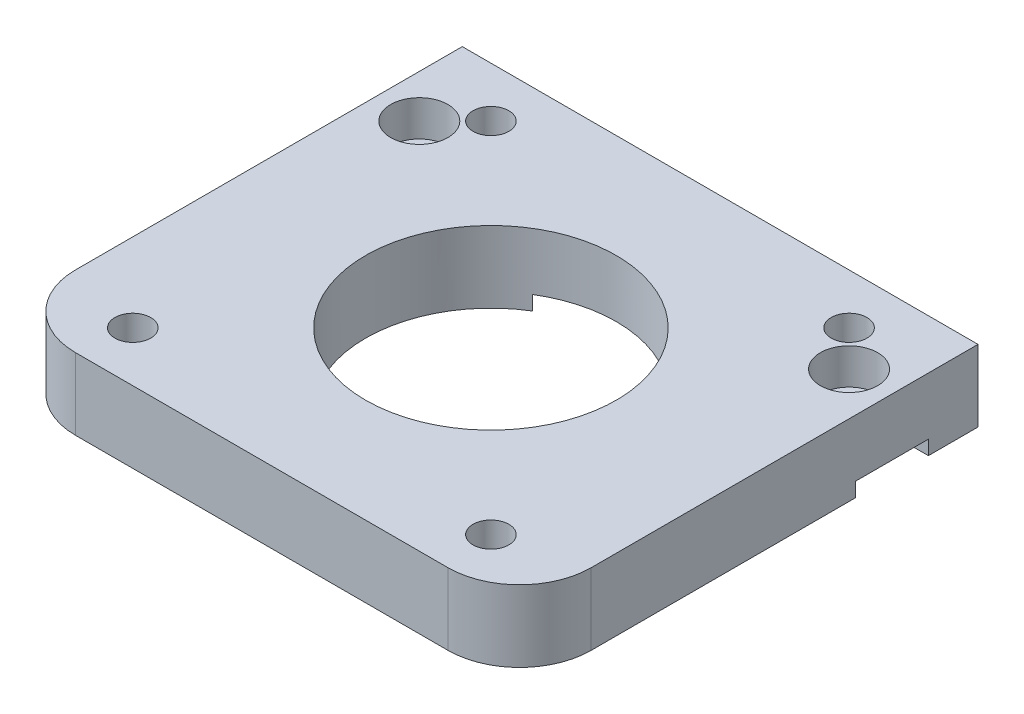
from build123d import *

# Parameters (mm, degrees)
SKETCH_1_W                = 103
SKETCH_1_H                = 100
EXTRUDE_1_DEPTH           = 10
SKETCH_9_W                = 15.5
SKETCH_9_H                = 88
CUT_EXTRUDE_4_DEPTH       = 144.906219463
HOLE_WIZARD_6_5_6_5_1_D   = 6.5
SKETCH_12_R               = 17.5
CUT_EXTRUDE_5_DEPTH       = 144.906219463
FILLET_1_R                = 10
HOLE_WIZARD_5_0_5_1_D     = 5
HOLE_WIZARD_5_0_5_1_DEPTH = 10
HOLE_WIZARD_5_0_5_1_TIP   = 1.502151548
FILLET_2_R                = 2
SKETCH_20_W               = 140.430498758
SKETCH_20_H               = 45.630669844
CUT_EXTRUDE_6_DEPTH       = 97
HOLE_WIZARD_1_D           = 4.4
HOLE_WIZARD_1_CBORE_D     = 8
HOLE_WIZARD_1_CBORE_DEPTH = 5
HOLE_WIZARD_M6_2_D        = 5
SKETCH_28_W               = 143.680703706
SKETCH_28_H               = 10.15
CUT_EXTRUDE_7_DEPTH       = 2


with BuildPart() as part:
    # 草图1 → 凸台-拉伸1 (new body)
    with BuildSketch(Plane(origin=(0, 0, 0), x_dir=(1, 0, 0), z_dir=(0, 1, 0))):
        with Locations((51.5, -50)):
            Rectangle(SKETCH_1_W, SKETCH_1_H)
    extrude(amount=EXTRUDE_1_DEPTH)

    # 草图9 → 切除-拉伸4 (cut, through all)
    with BuildSketch(Plane(origin=(0, 10, 0), x_dir=(1, 0, 0), z_dir=(0, 1, 0))):
        with Locations((7.75, -56)):
            Rectangle(SKETCH_9_W, SKETCH_9_H)
        with Locations((95.25, -56)):
            Rectangle(SKETCH_9_W, SKETCH_9_H)
    extrude(amount=-CUT_EXTRUDE_4_DEPTH, mode=Mode.SUBTRACT)

    # Ø6.5 (6.5) 直径孔1 (through all)
    with Locations(Plane.XY.offset(12)):
        with Locations((6, 5), (97, 5)):
            Hole(HOLE_WIZARD_6_5_6_5_1_D / 2)

    # 草图12 → 切除-拉伸5 (cut, through all)
    with BuildSketch(Plane(origin=(0, 10, 0), x_dir=(1, 0, 0), z_dir=(0, 1, 0))):
        with Locations(Location((51.5, -68, 0), (0, 0, 270))):
            Circle(SKETCH_12_R)
    extrude(amount=-CUT_EXTRUDE_5_DEPTH, mode=Mode.SUBTRACT)

    # 圆角1
    fillet_1_edges = [part.edges().sort_by_distance(p)[0] for p in [
        (15.5, 5, 100),
        (87.5, 5, 100),
    ]]
    fillet(fillet_1_edges, radius=FILLET_1_R)

    # Ø5.0 (5) 直径孔1
    with Locations(Plane(origin=(0, 0, 0), x_dir=(-1, 0, 0), z_dir=(0, 0, -1))):
        with Locations((-71.5, 5), (-31.5, 5)):
            Hole(HOLE_WIZARD_5_0_5_1_D / 2, depth=HOLE_WIZARD_5_0_5_1_DEPTH)
            with Locations((0, 0, -(HOLE_WIZARD_5_0_5_1_DEPTH + HOLE_WIZARD_5_0_5_1_TIP / 2))):  # 118° drill point
                Cone(0, HOLE_WIZARD_5_0_5_1_D / 2, HOLE_WIZARD_5_0_5_1_TIP, mode=Mode.SUBTRACT)

    # 圆角2
    fillet_2_edges = [part.edges().sort_by_distance(p)[0] for p in [
        (15.5, 5, 12),
        (87.5, 5, 12),
    ]]
    fillet(fillet_2_edges, radius=FILLET_2_R)

    # 草图20 → 切除-拉伸6 (cut)
    with BuildSketch(Plane(origin=(0, 10, 0), x_dir=(1, 0, 0), z_dir=(0, 1, 0))):
        with Locations((42.090220098, -13.184665078)):
            Rectangle(SKETCH_20_W, SKETCH_20_H)
    extrude(amount=-CUT_EXTRUDE_6_DEPTH, mode=Mode.SUBTRACT)

    # 打孔尺寸(%根据)内六角圆柱头螺钉的类型1 (through all)
    with Locations(Plane(origin=(0, 10, 0), x_dir=(1, 0, 0), z_dir=(0, 1, 0))):
        with Locations((21.5, -48), (81.5, -48)):
            CounterBoreHole(HOLE_WIZARD_1_D / 2, HOLE_WIZARD_1_CBORE_D / 2, HOLE_WIZARD_1_CBORE_DEPTH)

    # M6 螺纹孔2 (through all)
    with Locations(Plane(origin=(0, 10, 0), x_dir=(1, 0, 0), z_dir=(0, 1, 0))):
        with Locations((26.5, -43), (26.5, -93), (76.5, -93), (76.5, -43)):
            Hole(HOLE_WIZARD_M6_2_D / 2)

    # 草图28 → 切除-拉伸7 (cut)
    with BuildSketch(Plane.XZ):
        with Locations((21.5, 48)):
            Rectangle(SKETCH_28_W, SKETCH_28_H)
    extrude(amount=-CUT_EXTRUDE_7_DEPTH, mode=Mode.SUBTRACT)


solid = part.part
